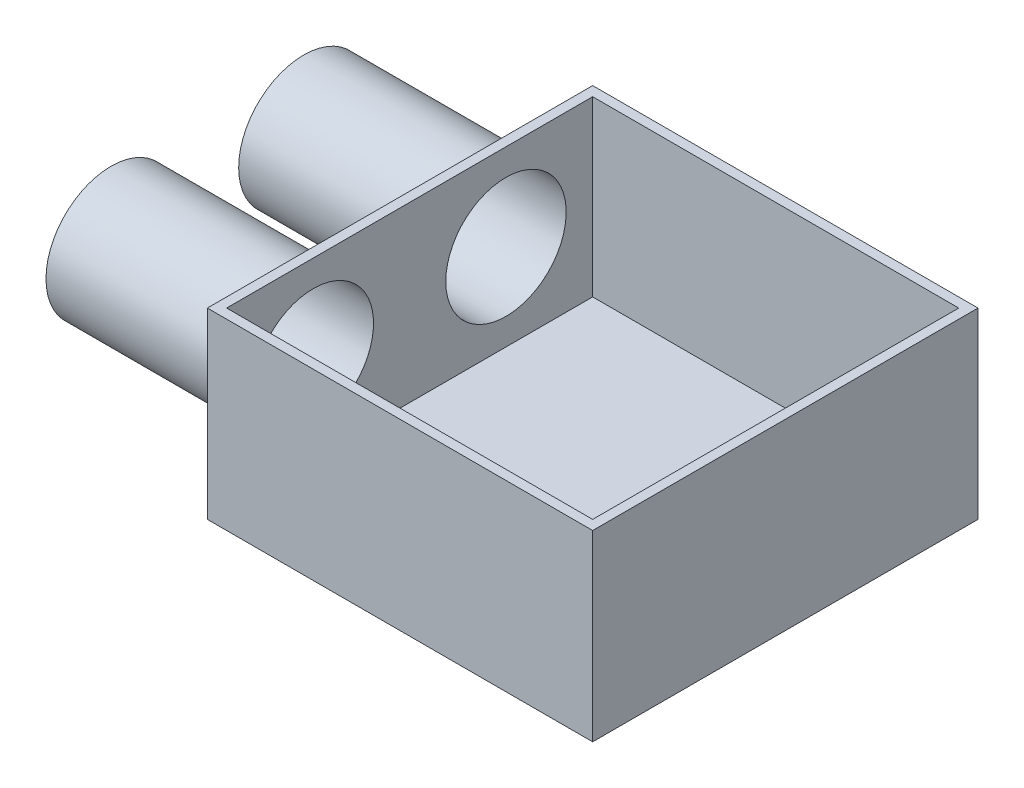
from build123d import *

# Parameters (mm, degrees)
SKETCH1_W           = 80
SKETCH1_H           = 80
BOSS_EXTRUDE1_DEPTH = 38
SKETCH2_W           = 76
SKETCH2_H           = 76
CUT_EXTRUDE1_DEPTH  = 36
SKETCH3_R           = 12.5
CUT_EXTRUDE2_DEPTH  = 10
BOSS_EXTRUDE3_START = 40
SKETCH4_R           = 13.5
SKETCH4_R_2         = 12.5
BOSS_EXTRUDE3_DEPTH = 40


with BuildPart() as part:
    # Sketch1 → Boss-Extrude1 (new body)
    with BuildSketch(Plane(origin=(0, 0, 0), x_dir=(1, 0, 0), z_dir=(0, 1, 0))):
        Rectangle(SKETCH1_W, SKETCH1_H)
    extrude(amount=BOSS_EXTRUDE1_DEPTH)

    # Sketch2 → Cut-Extrude1 (cut)
    with BuildSketch(Plane(origin=(0, 38, 0), x_dir=(1, 0, 0), z_dir=(0, 1, 0))):
        Rectangle(SKETCH2_W, SKETCH2_H)
    extrude(amount=-CUT_EXTRUDE1_DEPTH, mode=Mode.SUBTRACT)

    # Sketch3 → Cut-Extrude2 (cut)
    with BuildSketch(Plane.ZY.offset(40)):
        with Locations((-20, 20)):
            Circle(SKETCH3_R)
        with Locations((20, 20)):
            Circle(SKETCH3_R)
    extrude(amount=-CUT_EXTRUDE2_DEPTH, mode=Mode.SUBTRACT)

    # Sketch4 → Boss-Extrude3 (add)
    # profile 1 of 2: a face of its own
    with BuildSketch(Plane.ZY.offset(40).offset(BOSS_EXTRUDE3_START)):
        with Locations(Location((-20, 20, 0), (0, 0, 180))):
            Circle(SKETCH4_R)
        with Locations((-20, 20)):
            Circle(SKETCH4_R_2, mode=Mode.SUBTRACT)
    # profile 2 of 2: a face of its own
    with BuildSketch(Plane.ZY.offset(40).offset(BOSS_EXTRUDE3_START)):
        with Locations(Location((20, 20, 0), (0, 0, 180))):
            Circle(SKETCH4_R)
        with Locations((20, 20)):
            Circle(SKETCH4_R_2, mode=Mode.SUBTRACT)
    extrude(amount=-BOSS_EXTRUDE3_DEPTH)


solid = part.part
